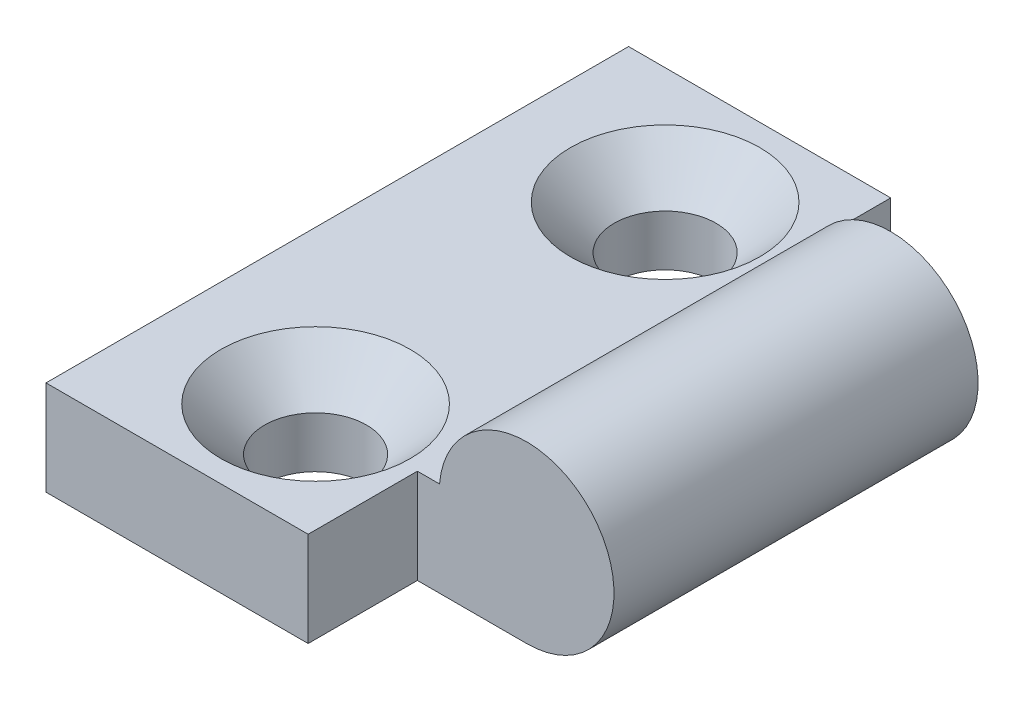
SolidWorks part; units mm, degrees
ref_plane "前视基准面" through (0, 0, 0) normal (0, 0, 1) x (1, 0, 0)
ref_plane "上视基准面" through (0, 0, 0) normal (0, 1, 0) x (1, 0, 0)
ref_plane "右视基准面" through (0, 0, 0) normal (1, 0, 0) x (0, 0, -1)
sketch "草图1" plane through (0, 0, 0) normal (0, 1, 0) x (1, 0, 0)
  line L1 (-12.75, 20) -> (12.75, 20)
  line L2 (-12.75, 20) -> (-12.75, -20)
  line L3 (-12.75, -20) -> (12.75, -20)
  line L4 (12.75, 20) -> (12.75, -20)
  line L5 (-12.75, 20) -> (12.75, -20) construction
  line L6 (-12.75, -20) -> (12.75, 20) construction
  point P0 (0, 0)
  dimension "D1" = 25.5
  dimension "D2" = 40
extrude "凸台-拉伸1" add sketch "草图1" along normal blind 6.5
sketch "草图2" plane through (0, 0, 20) normal (0, 0, 1) x (1, 0, 0)
  line L0 (-12.75, 0) -> (12.75, 0) construction
  line L1 (-12.75, 6.5) -> (-12.75, 0) construction
  circle A0 centre (12.75, 6) radius 6
  dimension "D1" = 25.5
  dimension "D2" = 12
extrude "凸台-拉伸2" add sketch "草图2" against normal up to surface (40 mm away) up to face at (0, 3.25, -20)
sketch "草图3" plane through (0, 0, 0) normal (0, -1, 0) x (1, 0, 0)
  line L0 (18.75, -20) -> (18.75, 20) construction
  line L1 (32.25, -12.5) -> (5.25, -12.5) construction
  line L2 (32.25, -12.5) -> (32.25, 12.5) construction
  line L3 (32.25, 12.5) -> (5.25, 12.5) construction
  line L4 (5.25, -12.5) -> (5.25, 12.5) construction
  line L5 (32.25, -12.5) -> (5.25, 12.5) construction
  line L6 (32.25, 12.5) -> (5.25, -12.5) construction
  line L8 (5.25, 12.5) -> (18.75, 12.5)
  line L9 (5.25, 12.5) -> (5.25, 20)
  line L10 (5.25, 20) -> (18.75, 20)
  line L11 (18.75, 12.5) -> (18.75, 20)
  line L12 (18.75, -20) -> (5.25, -20)
  line L13 (18.75, -20) -> (18.75, -12.5)
  line L14 (18.75, -12.5) -> (5.25, -12.5)
  line L15 (5.25, -20) -> (5.25, -12.5)
  point P0 (18.75, 0)
  dimension "D1" = 25
  dimension "D2" = 27
extrude "切除-拉伸1" cut sketch "草图3" against normal through all
sketch "草图5" plane through (0, 6.5, 0) normal (0, 1, 0) x (1, 0, 0)
  line L0 (0, 0) -> (37.6851, 0) construction
  line L2 (37.6851, 20.5307) -> (37.6851, -20.5307) construction
  line L3 (-2.2396, 12) -> (-2.2396, -12) construction
  line L4 (12.7604, 22) -> (12.7604, -12.5) construction
  line L5 (6.7709, -12.5) -> (18.75, -12.5) construction
  circle A0 centre (-2.2396, 12) radius 3.5
  circle A1 centre (-2.2396, -12) radius 3.5
  dimension "D3" = 7
  dimension "D1" = 24
  dimension "D2" = 15
extrude "切除-拉伸2" cut sketch "草图5" against normal through all
chamfer "倒角1" distance 3 angle 45 2 edges at (-2.2396, 6.5, 15.5) (-2.2396, 6.5, -8.5)
